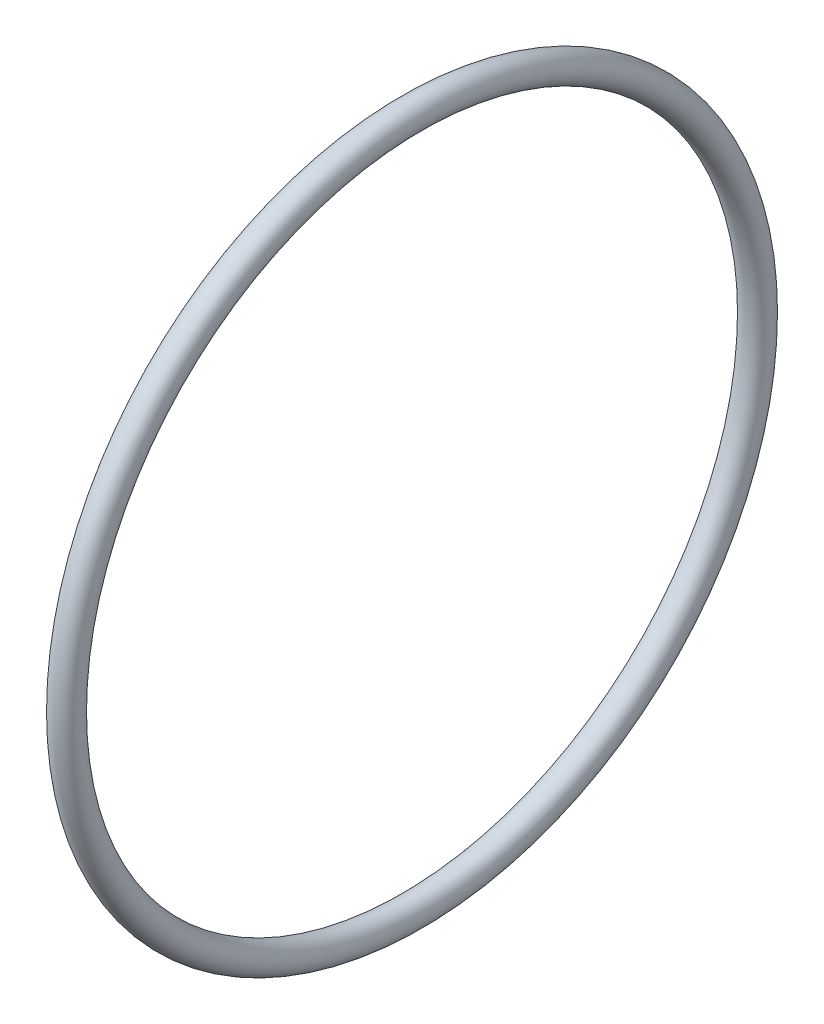
SolidWorks part; units mm, degrees
ref_plane "Front Plane" through (0, 0, 0) normal (0, 0, 1) x (1, 0, 0)
ref_plane "Top Plane" through (0, 0, 0) normal (0, 1, 0) x (1, 0, 0)
ref_plane "Right Plane" through (0, 0, 0) normal (1, 0, 0) x (0, 0, -1)
other "Configuration Table"
sketch "Sketch1" plane through (0, 0, 0) normal (0, 0, 1) x (1, 0, 0)
  line L0 (0, 0) -> (5, 0)
  circle A0 centre (5, 32.35) radius 1.325
  dimension "D2" = 2.65
  dimension "D1" = 5
  dimension "D3" = 32.35
revolve "Revolve1" add sketch "Sketch1" angle 360 about L0
